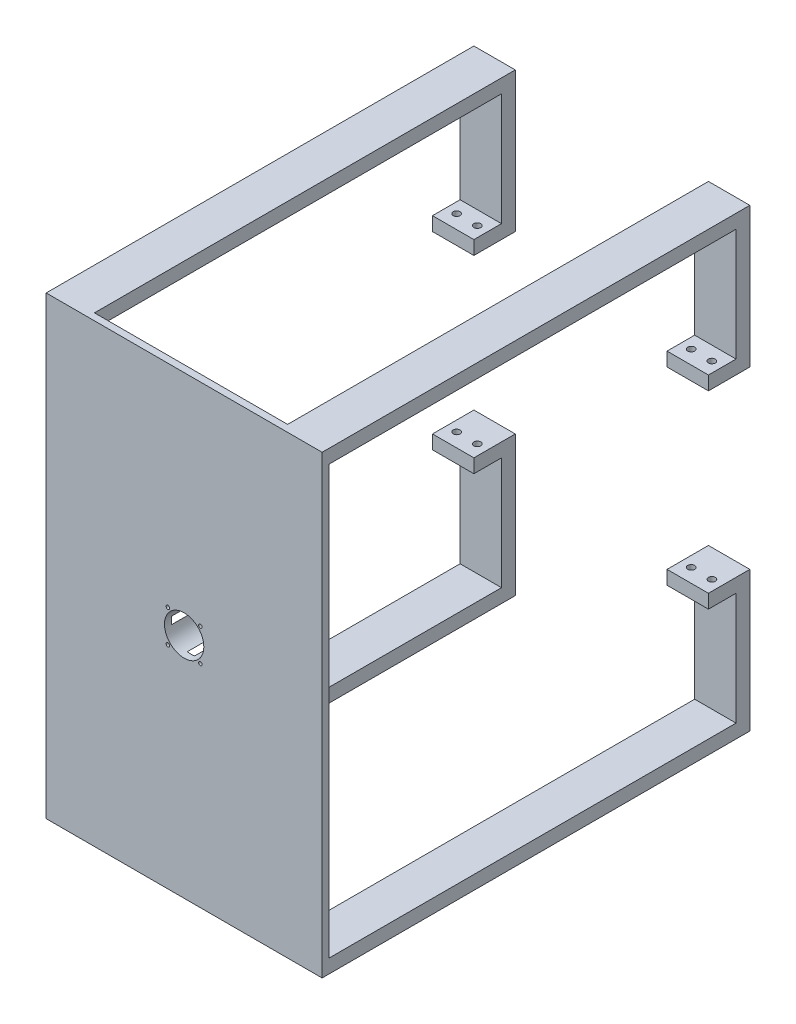
SolidWorks part; units mm, degrees
ref_plane "前视基准面" through (0, 0, 0) normal (0, 0, 1) x (1, 0, 0)
ref_plane "上视基准面" through (0, 0, 0) normal (0, 1, 0) x (1, 0, 0)
ref_plane "右视基准面" through (0, 0, 0) normal (1, 0, 0) x (0, 0, -1)
sketch "草图1" plane through (0, 0, 0) normal (0, 0, 1) x (1, 0, 0)
  line L1 (874.3578, 473.1203) -> (474.3578, 473.1203)
  line L2 (874.3578, 473.1203) -> (874.3578, -186.8797)
  line L3 (874.3578, -186.8797) -> (474.3578, -186.8797)
  line L4 (474.3578, 473.1203) -> (474.3578, -186.8797)
  line L5 (874.3578, 473.1203) -> (474.3578, -186.8797) construction
  line L6 (874.3578, -186.8797) -> (474.3578, 473.1203) construction
  circle A0 centre (674.3578, 143.1203) radius 28.5
  point P0 (674.3578, 143.1203)
  dimension "D1" = 57
  dimension "D2" = 660
  dimension "D3" = 400
  dimension "D4" = 660
extrude "凸台-拉伸1" add sketch "草图1" along normal blind 10
sketch "草图2" plane through (0, 0, -34.808) normal (0, 0, 1) x (1, 0, 0)
  line L8 (702.1219, 149.555) -> (701.3919, 167.7252)
  line L9 (696.7149, 172.041) -> (678.5447, 171.311)
  line L10 (667.9231, 170.8843) -> (649.7528, 170.1544)
  line L11 (645.4371, 165.4774) -> (646.167, 147.3071)
  line L12 (680.7925, 115.3562) -> (698.9628, 116.0861)
  line L13 (703.2785, 120.7631) -> (702.5486, 138.9334)
  line L14 (646.5937, 136.6855) -> (647.3237, 118.5153)
  line L15 (652.0007, 114.1995) -> (670.1709, 114.9295)
  arc A8 (702.1219, 149.555) -> (678.5447, 171.311) centre (674.3578, 143.1203) ccw
  arc A9 (701.3919, 167.7252) -> (696.7149, 172.041) centre (696.8956, 167.5446) ccw
  arc A10 (667.9231, 170.8843) -> (646.167, 147.3071) centre (674.3578, 143.1203) ccw
  arc A11 (649.7528, 170.1544) -> (645.4371, 165.4774) centre (649.9334, 165.658) ccw
  arc A12 (680.7925, 115.3562) -> (702.5486, 138.9334) centre (674.3578, 143.1203) ccw
  arc A13 (698.9628, 116.0861) -> (703.2785, 120.7631) centre (698.7821, 120.5825) ccw
  arc A14 (646.5937, 136.6855) -> (670.1709, 114.9295) centre (674.3578, 143.1203) ccw
  arc A15 (647.3237, 118.5153) -> (652.0007, 114.1995) centre (651.82, 118.6959) ccw
  circle A20 centre (696.9387, 167.5914) radius 2.6
  circle A21 centre (649.8867, 165.7012) radius 2.6
  circle A22 centre (651.7769, 118.6491) radius 2.6
  circle A23 centre (698.8289, 120.5393) radius 2.6
sketch "草图3" plane through (0, 0, 0) normal (0, 0, -1) x (-1, 0, 0)
  line L0 (-702.3578, 148.4353) -> (-702.3578, 166.6203) construction
  line L1 (-697.8578, 171.1203) -> (-679.6729, 171.1203) construction
  line L2 (-679.6729, 115.1203) -> (-697.8578, 115.1203) construction
  line L3 (-702.3578, 119.6203) -> (-702.3578, 137.8052) construction
  line L4 (-646.3578, 137.8052) -> (-646.3578, 119.6203) construction
  line L5 (-650.8578, 115.1203) -> (-669.0427, 115.1203) construction
  line L6 (-669.0427, 171.1203) -> (-650.8578, 171.1203) construction
  line L7 (-646.3578, 166.6203) -> (-646.3578, 148.4353) construction
  line L8 (-702.3578, 148.4353) -> (-702.3578, 166.6203)
  line L9 (-697.8578, 171.1203) -> (-679.6729, 171.1203)
  line L10 (-679.6729, 115.1203) -> (-697.8578, 115.1203)
  line L11 (-702.3578, 119.6203) -> (-702.3578, 137.8052)
  line L12 (-646.3578, 137.8052) -> (-646.3578, 119.6203)
  line L13 (-650.8578, 115.1203) -> (-669.0427, 115.1203)
  line L14 (-669.0427, 171.1203) -> (-650.8578, 171.1203)
  line L15 (-646.3578, 166.6203) -> (-646.3578, 148.4353)
  arc A0 (-679.6729, 171.1203) -> (-702.3578, 148.4353) centre (-674.3578, 143.1203) ccw construction
  arc A1 (-697.8578, 171.1203) -> (-702.3578, 166.6203) centre (-697.8578, 166.6203) ccw construction
  arc A2 (-702.3578, 137.8052) -> (-679.6729, 115.1203) centre (-674.3578, 143.1203) ccw construction
  arc A3 (-702.3578, 119.6203) -> (-697.8578, 115.1203) centre (-697.8578, 119.6203) ccw construction
  arc A4 (-669.0427, 115.1203) -> (-646.3578, 137.8052) centre (-674.3578, 143.1203) ccw construction
  arc A5 (-650.8578, 115.1203) -> (-646.3578, 119.6203) centre (-650.8578, 119.6203) ccw construction
  arc A6 (-646.3578, 148.4353) -> (-669.0427, 171.1203) centre (-674.3578, 143.1203) ccw construction
  arc A7 (-646.3578, 166.6203) -> (-650.8578, 171.1203) centre (-650.8578, 166.6203) ccw construction
  arc A8 (-679.6729, 171.1203) -> (-702.3578, 148.4353) centre (-674.3578, 143.1203) ccw
  arc A9 (-697.8578, 171.1203) -> (-702.3578, 166.6203) centre (-697.8578, 166.6203) ccw
  arc A10 (-702.3578, 137.8052) -> (-679.6729, 115.1203) centre (-674.3578, 143.1203) ccw
  arc A11 (-702.3578, 119.6203) -> (-697.8578, 115.1203) centre (-697.8578, 119.6203) ccw
  arc A12 (-669.0427, 115.1203) -> (-646.3578, 137.8052) centre (-674.3578, 143.1203) ccw
  arc A13 (-650.8578, 115.1203) -> (-646.3578, 119.6203) centre (-650.8578, 119.6203) ccw
  arc A14 (-646.3578, 148.4353) -> (-669.0427, 171.1203) centre (-674.3578, 143.1203) ccw
  arc A15 (-646.3578, 166.6203) -> (-650.8578, 171.1203) centre (-650.8578, 166.6203) ccw
extrude "凸台-拉伸3" add sketch "草图3" along normal blind 62.5
sketch "草图4" plane through (0, -186.8797, 0) normal (0, -1, 0) x (1, 0, 0)
  line L1 (474.3578, 10) -> (534.3578, 10)
  line L2 (474.3578, 10) -> (474.3578, -610)
  line L3 (474.3578, -610) -> (534.3578, -610)
  line L4 (534.3578, 10) -> (534.3578, -610)
  line L5 (874.3578, 10) -> (814.3578, 10)
  line L6 (874.3578, 10) -> (874.3578, -610)
  line L7 (874.3578, -610) -> (814.3578, -610)
  line L8 (814.3578, 10) -> (814.3578, -610)
  dimension "D1" = 60
  dimension "D2" = 60
  dimension "D3" = 620
extrude "凸台-拉伸4" add sketch "草图4" against normal blind 20
ref_plane "基准面1" through (0, 143.1203, 0) normal (0, -1, 0) x (-1, 0, 0)
mirror "镜向1" about plane through (0, 143.1203, 0) normal (0, -1, 0) of "凸台-拉伸4"
sketch "草图5" plane through (0, 473.1203, 0) normal (0, 1, 0) x (1, 0, 0)
  line L0 (814.3578, 0) -> (814.3578, 610) construction
  line L1 (874.3578, 610) -> (814.3578, 610)
  line L2 (874.3578, 610) -> (874.3578, 590)
  line L3 (874.3578, 590) -> (814.3578, 590)
  line L4 (814.3578, 610) -> (814.3578, 590)
  dimension "D1" = 20
extrude "凸台-拉伸5" add sketch "草图5" against normal blind 203
ref_plane "基准面2" through (674.3578, 0, 0) normal (1, 0, 0) x (0, 0, -1)
ref_plane "基准面3" through (0, 143.1203, 0) normal (0, -1, 0) x (-1, 0, 0)
mirror "镜向2" about plane through (674.3578, 0, 0) normal (1, 0, 0) of "凸台-拉伸5"
mirror "镜向3" about plane through (0, 143.1203, 0) normal (0, -1, 0) of "镜向2", "凸台-拉伸5" second plane through (674.3578, 0, 0) second plane normal (1, 0, 0)
sketch "草图6" plane through (0, 270.1203, 0) normal (0, -1, 0) x (1, 0, 0)
  line L0 (874.3578, -590) -> (874.3578, -610) construction
  line L1 (814.3578, -610) -> (874.3578, -610)
  line L2 (814.3578, -610) -> (814.3578, -550)
  line L3 (814.3578, -550) -> (874.3578, -550)
  line L4 (874.3578, -610) -> (874.3578, -550)
  dimension "D1" = 60
extrude "凸台-拉伸6" add sketch "草图6" against normal blind 20
mirror "镜向4" about plane through (674.3578, 0, 0) normal (1, 0, 0) of "凸台-拉伸6"
mirror "镜向5" about plane through (0, 143.1203, 0) normal (0, -1, 0) of "镜向4", "凸台-拉伸6"
sketch "草图7" plane through (0, 290.1203, 0) normal (0, 1, 0) x (1, 0, 0)
  line L0 (874.3578, 570) -> (814.3578, 570) construction
  line L1 (874.3578, 590) -> (874.3578, 550) construction
  line L2 (814.3578, 550) -> (814.3578, 590) construction
  circle A0 centre (859.3578, 570) radius 5
  circle A1 centre (829.3578, 570) radius 5
  dimension "D1" = 30
  dimension "D2" = 15
  dimension "D3" = 10
  dimension "D4" = 10
extrude "切除-拉伸1" cut sketch "草图7" against normal up to surface (294 mm away) up to face at (844.3578, -3.8797, -570)
mirror "镜向6" about plane through (674.3578, 0, 0) normal (1, 0, 0) of "切除-拉伸1"
sketch "草图8" plane through (0, 0, 10) normal (0, 0, 1) x (1, 0, 0)
  circle A4 centre (650.8128, 166.6653) radius 2.6
  circle A5 centre (650.8128, 119.5753) radius 2.6
  circle A6 centre (697.9028, 119.5753) radius 2.6
  circle A7 centre (697.9028, 166.6653) radius 2.6
extrude "切除-拉伸2" cut sketch "草图8" against normal through all
